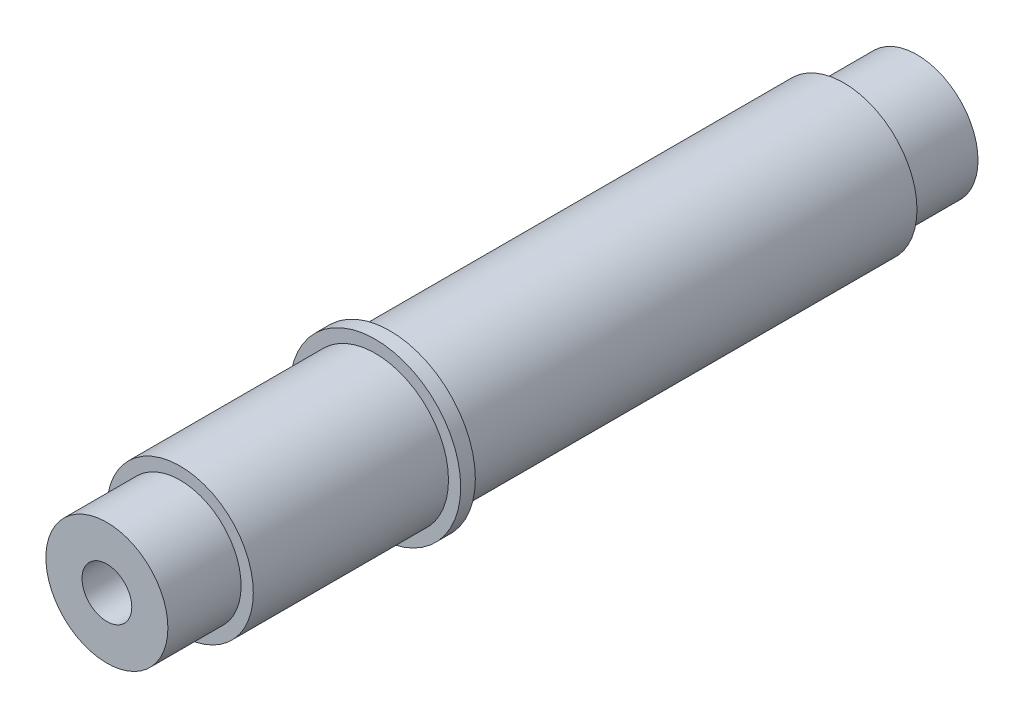
from build123d import *

# Parameters (mm, degrees)
SKETCH1_R              = 15
BOSS_EXTRUDE1_DEPTH    = 68
SKETCH2_R              = 12.5
BOSS_EXTRUDE2_DEPTH    = 15
BOSS_EXTRUDE4_START    = 25
SKETCH4_R              = 17.5
BOSS_EXTRUDE4_DEPTH    = 3
M12_TAPPED_HOLE1_D     = 10.2
M12_TAPPED_HOLE1_DEPTH = 32.75
M12_TAPPED_HOLE1_TIP   = 3.064389157
M12_TAPPED_HOLE2_D     = 10.2
M12_TAPPED_HOLE2_DEPTH = 32.75
M12_TAPPED_HOLE2_TIP   = 3.064389157


with BuildPart() as part:
    # Sketch1 → Boss-Extrude1 (new, symmetric)
    with BuildSketch(Plane.XY):
        Circle(SKETCH1_R)
    extrude(amount=BOSS_EXTRUDE1_DEPTH, both=True)

    # Sketch2 → Boss-Extrude2 (add)
    with BuildSketch(Plane.XY.offset(68)):
        Circle(SKETCH2_R)
    boss_extrude2 = extrude(amount=BOSS_EXTRUDE2_DEPTH)

    # Mirror1: Boss-Extrude2 across plane
    add(boss_extrude2.mirror(Plane.XY))

    # Sketch4 → Boss-Extrude4 (add)
    with BuildSketch(Plane.XY.offset(BOSS_EXTRUDE4_START)):
        Circle(SKETCH4_R)
    extrude(amount=BOSS_EXTRUDE4_DEPTH)

    # M12 Tapped Hole1
    with Locations(Plane(origin=(0, 0, -83), x_dir=(-1, 0, 0), z_dir=(0, 0, -1))):
        with Locations((0, 0)):
            Hole(M12_TAPPED_HOLE1_D / 2, depth=M12_TAPPED_HOLE1_DEPTH)
            with Locations((0, 0, -(M12_TAPPED_HOLE1_DEPTH + M12_TAPPED_HOLE1_TIP / 2))):  # 118° drill point
                Cone(0, M12_TAPPED_HOLE1_D / 2, M12_TAPPED_HOLE1_TIP, mode=Mode.SUBTRACT)

    # M12 Tapped Hole2
    with Locations(Plane.XY.offset(83)):
        with Locations((0, 0)):
            Hole(M12_TAPPED_HOLE2_D / 2, depth=M12_TAPPED_HOLE2_DEPTH)
            with Locations((0, 0, -(M12_TAPPED_HOLE2_DEPTH + M12_TAPPED_HOLE2_TIP / 2))):  # 118° drill point
                Cone(0, M12_TAPPED_HOLE2_D / 2, M12_TAPPED_HOLE2_TIP, mode=Mode.SUBTRACT)


solid = part.part
